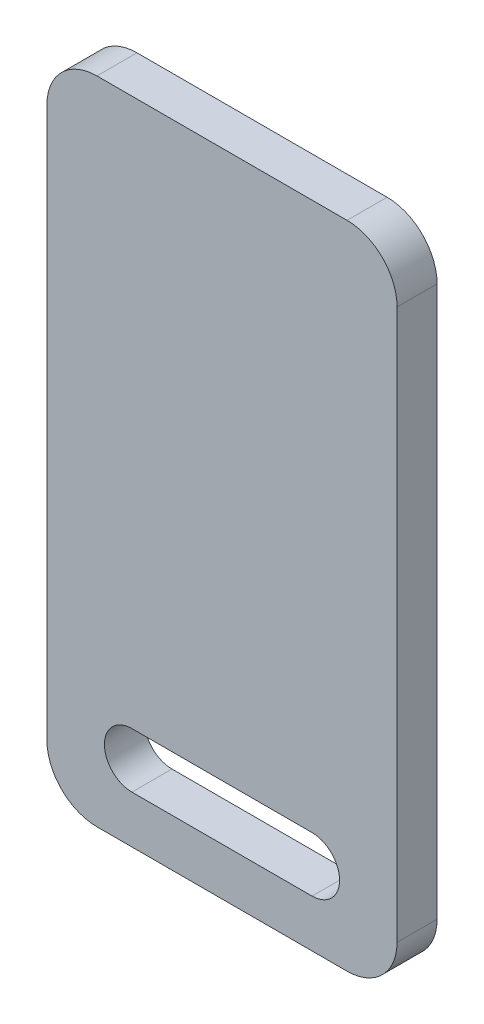
SolidWorks part; units mm, degrees
material "Q235"
ref_plane "Front Plane" through (0, 0, 0) normal (0, 0, 1) x (1, 0, 0)
ref_plane "Top Plane" through (0, 0, 0) normal (0, 1, 0) x (1, 0, 0)
ref_plane "Right Plane" through (0, 0, 0) normal (1, 0, 0) x (0, 0, -1)
sketch "Sketch1" plane through (0, 0, 0) normal (0, 0, 1) x (1, 0, 0)
  line L1 (10, 0) -> (60, 0)
  line L2 (0, 10) -> (0, 120)
  line L3 (10, 130) -> (60, 130)
  line L4 (70, 10) -> (70, 120)
  arc A2 (70, 120) -> (60, 130) centre (60, 120) ccw
  arc A3 (10, 130) -> (0, 120) centre (10, 120) ccw
  arc A4 (70, 10) -> (60, 0) centre (60, 10) cw
  arc A5 (10, 0) -> (0, 10) centre (10, 10) cw
  point P17 (0, 130)
  point P20 (70, 0)
  point P23 (0, 0)
  dimension "D7" = 10
  dimension "D1" = 70
  dimension "D2" = 130
extrude "Boss-Extrude1" add sketch "Sketch1" along normal blind 8
sketch "Sketch2" plane through (0, 0, 8) normal (0, 0, 1) x (1, 0, 0)
  line L0 (17, 15) -> (53, 15) construction
  line L1 (17, 20.5) -> (53, 20.5)
  line L2 (17, 9.5) -> (53, 9.5)
  line L3 (10, 0) -> (60, 0) construction
  line L4 (35, 0) -> (35, 15) construction
  arc A0 (17, 20.5) -> (17, 9.5) centre (17, 15) ccw
  arc A1 (53, 9.5) -> (53, 20.5) centre (53, 15) ccw
  point P2 (35, 15)
  dimension "D1" = 15
  dimension "D2" = 11
  dimension "D3" = 36
extrude "Cut-Extrude1" cut sketch "Sketch2" against normal blind 10
